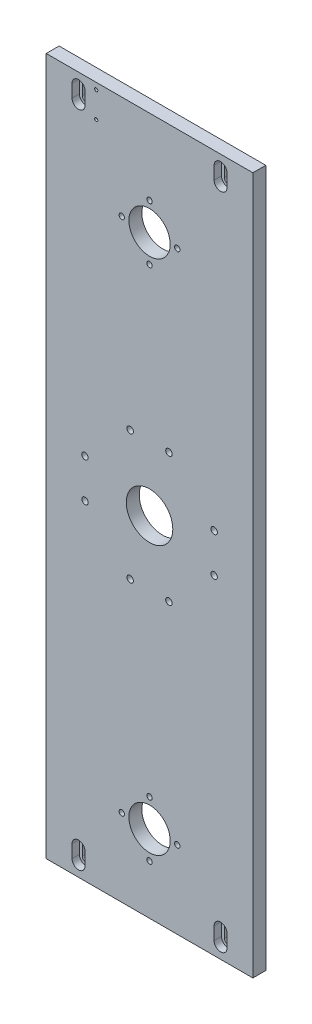
SolidWorks part; units mm, degrees
ref_plane "前视基准面" through (0, 0, 0) normal (0, 0, 1) x (1, 0, 0)
ref_plane "上视基准面" through (0, 0, 0) normal (0, 1, 0) x (1, 0, 0)
ref_plane "右视基准面" through (0, 0, 0) normal (1, 0, 0) x (0, 0, -1)
sketch "草图1" plane through (0, 0, 0) normal (0, 0, 1) x (1, 0, 0)
  line L1 (80, 270) -> (-80, 270)
  line L2 (80, 270) -> (80, -270)
  line L3 (80, -270) -> (-80, -270)
  line L4 (-80, 270) -> (-80, -270)
  line L5 (80, 270) -> (-80, -270) construction
  line L6 (80, -270) -> (-80, 270) construction
  point P0 (0, 0)
  dimension "D1" = 540
  dimension "D2" = 160
extrude "凸台-拉伸1" add sketch "草图1" along normal blind 10
sketch "草图2" plane through (0, 0, 10) normal (0, 0, 1) x (1, 0, 0)
  line L0 (80, 270) -> (-80, 270) construction
  line L1 (-80, -270) -> (80, -270) construction
  circle A0 centre (0, 190) radius 16
  circle A1 centre (0, -210) radius 16
  dimension "D1" = 32
  dimension "D2" = 32
  dimension "D3" = 80
  dimension "D4" = 60
extrude "切除-拉伸1" cut sketch "草图2" against normal through all
sketch "草图3" plane through (0, 0, 10) normal (0, 0, 1) x (1, 0, 0)
  line L0 (-80, 270) -> (-80, -270) construction
  line L1 (80, 270) -> (-80, 270) construction
  circle A0 centre (0, 0) radius 18
  dimension "D2" = 36
  dimension "D1" = 80
  dimension "D3" = 270
extrude "切除-拉伸2" cut sketch "草图3" against normal through all
hole_wizard "打孔尺寸根据内六角圆柱头螺钉的类型1" positions "草图7" profile "草图6" counterbore size "M5" standard "Gb" end condition through all
sketch "草图7" plane through (0, 0, 10) normal (0, 0, 1) x (1, 0, 0)
  line L0 (80, 270) -> (-80, 270) construction
  line L1 (-80, -270) -> (80, -270) construction
  line L2 (-80, 270) -> (-80, -270) construction
  line L3 (80, -270) -> (80, 270) construction
  point P0 (-55, 255)
  point P2 (55, 255)
  point P4 (55, -255)
  point P6 (-55, -255)
  dimension "D1" = 15
  dimension "D2" = 15
  dimension "D3" = 15
  dimension "D4" = 15
  dimension "D5" = 25
  dimension "D6" = 25
  dimension "D7" = 25
  dimension "D8" = 25
sketch "草图6" plane through (-55, 255, 10) normal (1, 0, 0) x (0, -1, 0)
  line L0 (0, 0) -> (0, 10)
  line L1 (0, 10) -> (2.75, 10)
  line L3 (2.75, 10) -> (2.75, 5.7)
  line L4 (2.75, 5.7) -> (5, 5.7)
  line L5 (5, 5.7) -> (5, 0)
  line L7 (5, 0) -> (0, 0)
  line L11 (0, -6.35) -> (0, 107.95) construction
  dimension "通孔孔直径" = 5.5
  dimension "通孔孔深度" = 10
  dimension "柱形沉头孔直径" = 10
  dimension "柱形沉头孔深度" = 5.7
hole_wizard "M5 螺纹孔1" positions "草图12" profile "草图11" tap size "M5" standard "Iso" end condition through all
sketch "草图12" plane through (0, 0, 10) normal (0, 0, 1) x (1, 0, 0)
  line L0 (80, 270) -> (-80, 270) construction
  point P0 (0, 211.5)
  dimension "D1" = 58.5
cosmetic thread "孔螺蚊线5" parameters "D2"=5
sketch "草图11" plane through (0, 211.5, 10) normal (1, 0, 0) x (0, -1, 0)
  line L0 (0, 0) -> (0, 10)
  line L1 (0, 10) -> (2.1, 10)
  line L2 (2.1, 10) -> (2.1, 0)
  line L5 (2.1, 0) -> (0, 0)
  line L11 (0, -6.35) -> (0, 107.95) construction
  dimension "通孔螺纹孔钻头直径" = 4.2
  dimension "通孔螺纹孔钻头深度" = 10
hole_wizard "M5 螺纹孔2" positions "草图14" profile "草图13" tap size "M5" standard "Iso" end condition through all
sketch "草图14" plane through (0, 0, 10) normal (0, 0, 1) x (1, 0, 0)
  line L0 (-80, -270) -> (80, -270) construction
  point P0 (0, -231.5)
  dimension "D1" = 38.5
cosmetic thread "孔螺蚊线6" parameters "D2"=5
sketch "草图13" plane through (0, -231.5, 10) normal (1, 0, 0) x (0, -1, 0)
  line L0 (0, 0) -> (0, 10)
  line L1 (0, 10) -> (2.1, 10)
  line L2 (2.1, 10) -> (2.1, 0)
  line L5 (2.1, 0) -> (0, 0)
  line L11 (0, -6.35) -> (0, 107.95) construction
  dimension "通孔螺纹孔钻头直径" = 4.2
  dimension "通孔螺纹孔钻头深度" = 10
hole_wizard "M5 螺纹孔3" positions "草图16" profile "草图15" tap size "M5" standard "Iso" end condition through all
sketch "草图16" plane through (0, 0, 10) normal (0, 0, 1) x (1, 0, 0)
  point P0 (21.5, -210)
  point P3 (-21.5, -210)
  point P6 (0, -188.5)
  point P9 (-21.5, 190)
  point P12 (21.5, 190)
  point P15 (0, 168.5)
sketch "草图15" plane through (21.5, -210, 10) normal (1, 0, 0) x (0, -1, 0)
  line L0 (0, 0) -> (0, 10)
  line L1 (0, 10) -> (2.1, 10)
  line L2 (2.1, 10) -> (2.1, 0)
  line L5 (2.1, 0) -> (0, 0)
  line L11 (0, -6.35) -> (0, 107.95) construction
  dimension "通孔螺纹孔钻头直径" = 4.2
  dimension "通孔螺纹孔钻头深度" = 10
cosmetic thread "孔螺蚊线7" parameters "D2"=5
cosmetic thread "孔螺蚊线8" parameters "D2"=5
cosmetic thread "孔螺蚊线9" parameters "D2"=5
cosmetic thread "孔螺蚊线10" parameters "D2"=5
cosmetic thread "孔螺蚊线11" parameters "D2"=5
cosmetic thread "孔螺蚊线12" parameters "D2"=5
hole_wizard "M3 螺纹孔1" positions "草图18" profile "草图17" tap size "M3" standard "Iso" end condition through all
sketch "草图18" plane through (0, 0, 10) normal (0, 0, 1) x (1, 0, 0)
  line L0 (-80, 270) -> (-80, -270) construction
  line L1 (80, 270) -> (-80, 270) construction
  point P0 (-41.3, 265)
  point P3 (-41.3, 245)
  dimension "D1" = 38.7
  dimension "D2" = 38.7
  dimension "D3" = 5
  dimension "D4" = 25
sketch "草图17" plane through (-41.3, 265, 10) normal (1, 0, 0) x (0, -1, 0)
  line L0 (0, 0) -> (0, 10)
  line L1 (0, 10) -> (1.25, 10)
  line L2 (1.25, 10) -> (1.25, 0)
  line L5 (1.25, 0) -> (0, 0)
  line L11 (0, -6.35) -> (0, 107.95) construction
  dimension "通孔螺纹孔钻头直径" = 2.5
  dimension "通孔螺纹孔钻头深度" = 10
cosmetic thread "孔螺蚊线13" parameters "D2"=3
cosmetic thread "孔螺蚊线14" parameters "D2"=3
sketch "草图21" plane through (0, 0, 0) normal (0, 0, -1) x (-1, 0, 0)
  line L1 (-50, 15) -> (50, 15)
  line L2 (-50, 15) -> (-50, -15)
  line L3 (-50, -15) -> (50, -15)
  line L4 (50, 15) -> (50, -15)
  line L5 (-50, 15) -> (50, -15) construction
  line L6 (-50, -15) -> (50, 15) construction
  point P0 (0, 0)
  dimension "D1" = 30
  dimension "D2" = 100
hole_wizard "M6 螺纹孔2" positions "草图23" profile "草图22" tap size "M6" standard "Iso" end condition through all
sketch "草图23" plane through (0, 0, 0) normal (0, 0, -1) x (-1, 0, 0)
  point P0 (-50, 15)
  point P3 (-50, -15)
  point P6 (50, 15)
  point P9 (50, -15)
sketch "草图22" plane through (50, 15, 0) normal (1, 0, 0) x (0, 1, 0)
  line L0 (0, 0) -> (0, 10)
  line L1 (0, 10) -> (2.5, 10)
  line L2 (2.5, 10) -> (2.5, 0)
  line L5 (2.5, 0) -> (0, 0)
  line L11 (0, -6.35) -> (0, 107.95) construction
  dimension "通孔螺纹孔钻头直径" = 5
  dimension "通孔螺纹孔钻头深度" = 10
cosmetic thread "孔螺蚊线19" parameters "D2"=6
cosmetic thread "孔螺蚊线20" parameters "D2"=6
cosmetic thread "孔螺蚊线21" parameters "D2"=6
cosmetic thread "孔螺蚊线22" parameters "D2"=6
sketch "草图24" plane through (0, 0, 10) normal (0, 0, 1) x (1, 0, 0)
  line L0 (-55, 260) -> (-55, 250) construction
  line L1 (-50, 260) -> (-50, 250)
  line L2 (-60, 260) -> (-60, 250)
  line L3 (55, 260) -> (55, 250) construction
  line L4 (60, 260) -> (60, 250)
  line L5 (50, 260) -> (50, 250)
  line L6 (-55, -250) -> (-55, -260) construction
  line L7 (-50, -250) -> (-50, -260)
  line L8 (-60, -250) -> (-60, -260)
  line L9 (55, -250) -> (55, -260) construction
  line L10 (60, -250) -> (60, -260)
  line L11 (50, -250) -> (50, -260)
  circle A0 centre (-55, 255) radius 5 construction
  circle A1 centre (-55, 255) radius 5 construction
  arc A2 (-50, 260) -> (-60, 260) centre (-55, 260) ccw
  arc A3 (-60, 250) -> (-50, 250) centre (-55, 250) ccw
  circle A4 centre (55, 255) radius 5 construction
  circle A5 centre (55, 255) radius 5 construction
  arc A6 (60, 260) -> (50, 260) centre (55, 260) ccw
  arc A7 (50, 250) -> (60, 250) centre (55, 250) ccw
  circle A8 centre (-55, -255) radius 5 construction
  arc A9 (-50, -250) -> (-60, -250) centre (-55, -250) ccw
  arc A10 (-60, -260) -> (-50, -260) centre (-55, -260) ccw
  circle A11 centre (55, -255) radius 5 construction
  circle A12 centre (55, -255) radius 5 construction
  arc A13 (60, -250) -> (50, -250) centre (55, -250) ccw
  arc A14 (50, -260) -> (60, -260) centre (55, -260) ccw
  point P7 (-55, 255)
  point P19 (55, 255)
  point P29 (-55, -255)
  point P34 (55, -255)
  dimension "D1" = 5
  dimension "D2" = 5
  dimension "D3" = 5
extrude "切除-拉伸3" cut sketch "草图24" against normal blind 5.7
sketch "草图25" plane through (0, 0, 4.3) normal (0, 0, 1) x (1, 0, 0)
  line L0 (-55, 260) -> (-55, 250) construction
  line L1 (-52.25, 260) -> (-52.25, 250)
  line L2 (-57.75, 260) -> (-57.75, 250)
  line L3 (55, 260) -> (55, 250) construction
  line L4 (57.75, 260) -> (57.75, 250)
  line L5 (52.25, 260) -> (52.25, 250)
  line L6 (-55, -250) -> (-55, -260) construction
  line L7 (-52.25, -250) -> (-52.25, -260)
  line L8 (-57.75, -250) -> (-57.75, -260)
  line L9 (55, -250) -> (55, -260) construction
  line L10 (57.75, -250) -> (57.75, -260)
  line L11 (52.25, -250) -> (52.25, -260)
  arc A0 (-52.25, 260) -> (-57.75, 260) centre (-55, 260) ccw
  arc A1 (-57.75, 250) -> (-52.25, 250) centre (-55, 250) ccw
  arc A2 (57.75, 260) -> (52.25, 260) centre (55, 260) ccw
  arc A3 (52.25, 250) -> (57.75, 250) centre (55, 250) ccw
  arc A4 (-52.25, -250) -> (-57.75, -250) centre (-55, -250) ccw
  arc A5 (-57.75, -260) -> (-52.25, -260) centre (-55, -260) ccw
  arc A6 (57.75, -250) -> (52.25, -250) centre (55, -250) ccw
  arc A7 (52.25, -260) -> (57.75, -260) centre (55, -260) ccw
  point P4 (-55, 255)
  point P11 (55, 255)
  point P18 (-55, -255)
  point P27 (55, -255)
extrude "切除-拉伸4" cut sketch "草图25" against normal through all
hole_wizard "M6 螺纹孔3" positions "草图27" profile "草图26" tap size "M6" standard "Iso" end condition through all
sketch "草图27" plane through (0, 0, 0) normal (0, 0, -1) x (-1, 0, 0)
  point P0 (15, -50)
  point P3 (-15, -50)
  point P6 (-15, 50)
  point P9 (15, 50)
cosmetic thread "孔螺蚊线23" parameters "D2"=6
cosmetic thread "孔螺蚊线24" parameters "D2"=6
cosmetic thread "孔螺蚊线25" parameters "D2"=6
cosmetic thread "孔螺蚊线26" parameters "D2"=6
sketch "草图26" plane through (-15, -50, 0) normal (1, 0, 0) x (0, 1, 0)
  line L0 (0, 0) -> (0, 10)
  line L1 (0, 10) -> (2.5, 10)
  line L2 (2.5, 10) -> (2.5, 0)
  line L5 (2.5, 0) -> (0, 0)
  line L11 (0, -6.35) -> (0, 107.95) construction
  dimension "通孔螺纹孔钻头直径" = 5
  dimension "通孔螺纹孔钻头深度" = 10
